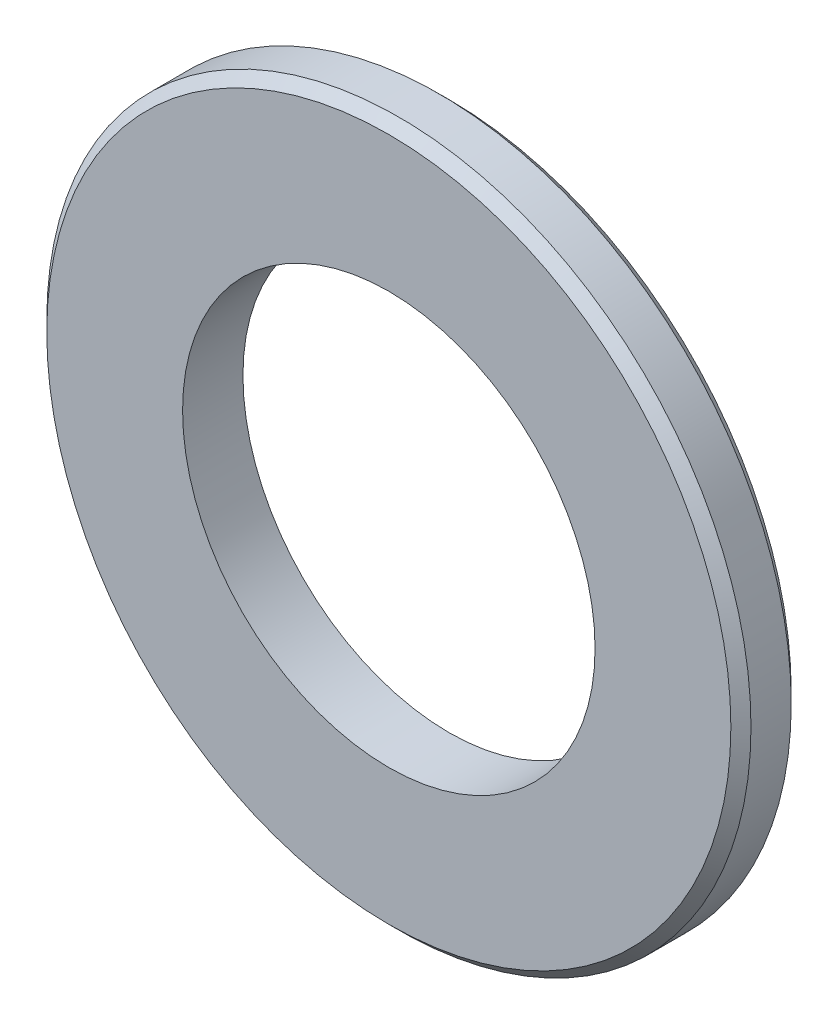
SolidWorks part; units mm, degrees
ref_plane "前视基准面" through (0, 0, 0) normal (0, 0, 1) x (1, 0, 0)
ref_plane "上视基准面" through (0, 0, 0) normal (0, 1, 0) x (1, 0, 0)
ref_plane "右视基准面" through (0, 0, 0) normal (1, 0, 0) x (0, 0, -1)
sketch "草图1" plane through (0, 0, 0) normal (0, 0, 1) x (1, 0, 0)
  circle A0 centre (0, 0) radius 17.5
  circle A1 centre (0, 0) radius 10.25
  dimension "D1" = 35
  dimension "D2" = 20.5
extrude "凸台-拉伸1" add sketch "草图1" along normal blind 3
chamfer "倒角1" distance 0.5 angle 45 2 edges at (17.5, 0, 0) (17.5, 0, 3)
